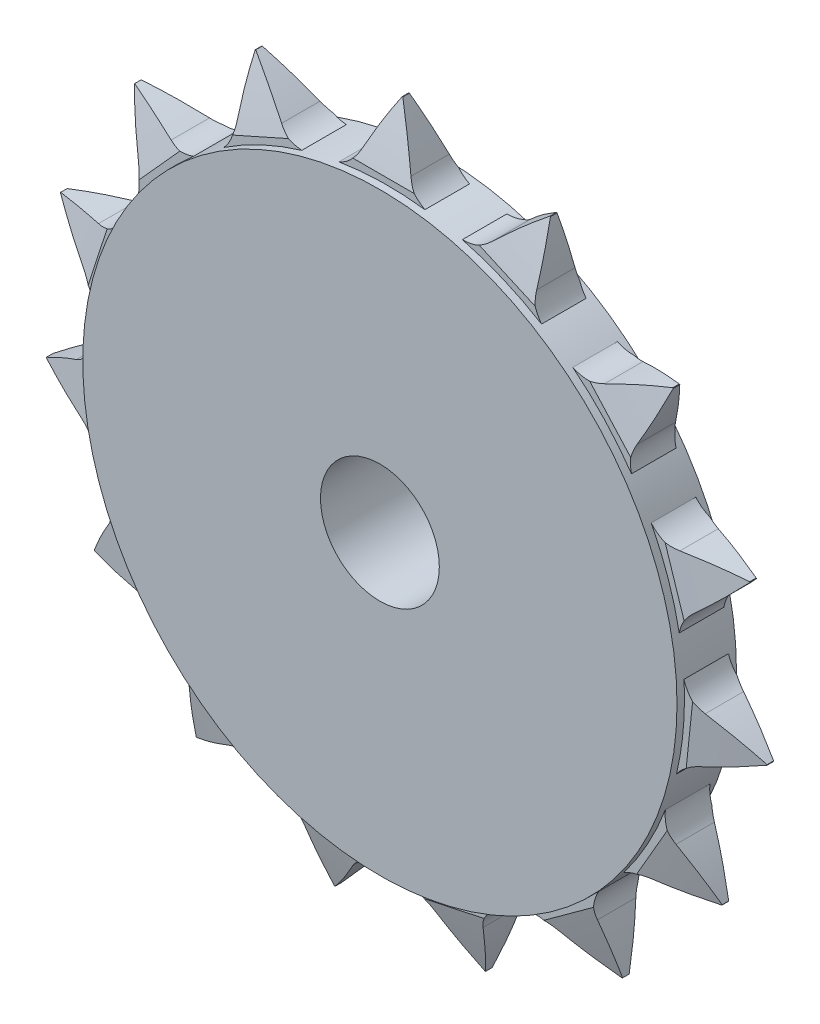
SolidWorks part; units mm, degrees
ref_plane "Front Plane" through (0, 0, 0) normal (0, 0, 1) x (1, 0, 0)
ref_plane "Top Plane" through (0, 0, 0) normal (0, 1, 0) x (1, 0, 0)
ref_plane "Right Plane" through (0, 0, 0) normal (1, 0, 0) x (0, 0, -1)
sketch "Sketch1" plane through (0, 0, 0) normal (0, 0, 1) x (1, 0, 0)
  circle A0 centre (0, 0) radius 5
  dimension "D1" = 10
extrude "Boss-Extrude1" add sketch "Sketch1" along normal blind 1
sketch "Sketch2" plane through (0, 0, 0) normal (0, 0, -1) x (-1, 0, 0)
  circle A0 centre (0, 0) radius 3.8118
extrude "Boss-Extrude2" add sketch "Sketch2" along normal blind 0.75
ref_plane "Plane1" through (0, 0, 0.5) normal (0, 0, 1) x (1, 0, 0)
sketch "Sketch5" plane through (0, 0, 0.5) normal (0, 0, 1) x (1, 0, 0)
  line L0 (-0.069, 6.0972) -> (-0.059, 6.0972)
  line L1 (-0.064, 6.0972) -> (-0.064, 4.9418) construction
  arc A0 (-0.069, 6.0972) -> (-0.4735, 5.2762) centre (6.005, 2.5949) ccw
  arc A1 (-0.9873, 4.8877) -> (-0.4735, 5.2762) centre (-1.0611, 5.5194) ccw
  arc A2 (0.8593, 4.889) -> (0.3454, 5.2762) centre (0.9325, 5.5207) cw
  arc A3 (-0.059, 6.0972) -> (0.3454, 5.2762) centre (-7.817, 1.7653) cw
  arc A4 (0.8593, 4.889) -> (-0.9873, 4.8877) centre (-0.0585, -3.0586) ccw
  dimension "D1" = 0.01
extrude "Boss-Extrude3" add sketch "Sketch5" along normal mid plane 0.75
sketch "Sketch7" plane through (0, 0, 0) normal (1, 0, 0) x (0, 0, -1)
  line L0 (-0.55, 6.1112) -> (-0.45, 6.1112)
  line L1 (-0.125, 5.1047) -> (0.244, 5.1047)
  line L2 (0.244, 5.1047) -> (0.244, 6.4606)
  line L3 (0.244, 6.4606) -> (-1.1669, 6.4606)
  line L4 (-1.1669, 6.4606) -> (-1.1669, 5.1047)
  line L5 (-1.1669, 5.1047) -> (-0.875, 5.1047)
  line L6 (-0.5, 6.0972) -> (-0.5, 6.1112) construction
  line L7 (-0.875, 6.0972) -> (-0.125, 6.0972) construction
  line L8 (-0.125, 4.9332) -> (-0.125, 5.2762) construction
  line L9 (-0.875, 5.2762) -> (-0.875, 4.9332) construction
  arc A0 (-0.875, 5.1047) -> (-0.55, 6.1112) centre (23.0726, -2.0724) cw
  arc A1 (-0.125, 5.1047) -> (-0.45, 6.1112) centre (-24.0726, -2.0724) ccw
  dimension "D1" = 25
  dimension "D2" = 0.1
extrude "Cut-Extrude1" cut sketch "Sketch7" against normal through all both and the other way through all
pattern_circular "CirPattern1" count 15 over 360 about axis through (0, 0, 0) along (0, 0, 1) of "Boss-Extrude3", "Cut-Extrude1"
sketch "Sketch8" plane through (0, 0, -0.75) normal (0, 0, -1) x (-1, 0, 0)
  circle A0 centre (0, 0) radius 1
  dimension "D1" = 2
extrude "Cut-Extrude2" cut sketch "Sketch8" against normal blind 20.75
